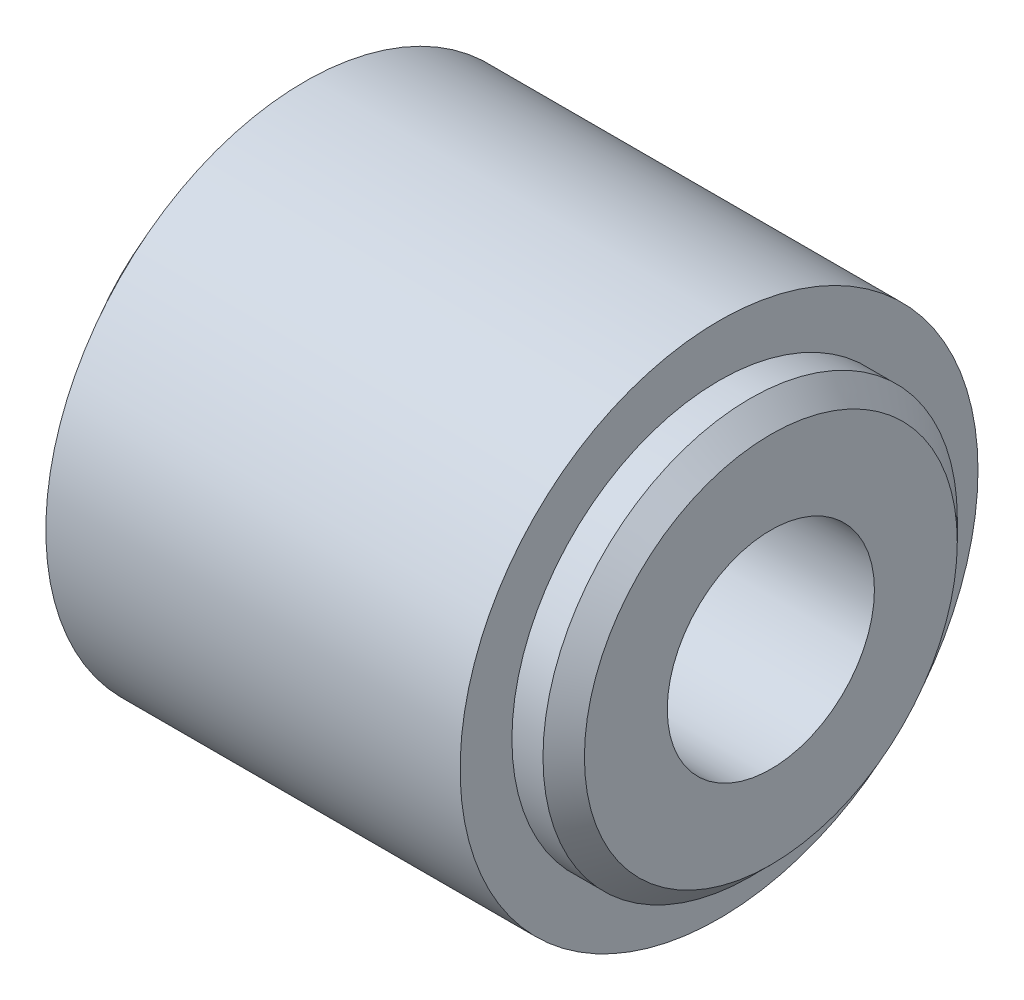
from build123d import *

# Parameters (mm, degrees)
SKETCH_1_R      = 10
SKETCH_1_R_2    = 5
EXTRUDE_1_DEPTH = 12.5
SKETCH_2_R      = 12.5
SKETCH_2_R_2    = 10
EXTRUDE_2_DEPTH = 10
CHAMFER_1_SIZE  = 1


with BuildPart() as part:
    # 草图1 → 凸台-拉伸1 (new, symmetric)
    with BuildSketch(Plane(origin=(0, 0, 0), x_dir=(0, 0, -1), z_dir=(1, 0, 0))):
        Circle(SKETCH_1_R)
        Circle(SKETCH_1_R_2, mode=Mode.SUBTRACT)
    extrude(amount=EXTRUDE_1_DEPTH, both=True)

    # 草图2 → 凸台-拉伸2 (add, symmetric)
    with BuildSketch(Plane(origin=(0, 0, 0), x_dir=(0, 0, -1), z_dir=(1, 0, 0))):
        Circle(SKETCH_2_R)
        Circle(SKETCH_2_R_2, mode=Mode.SUBTRACT)
    extrude(amount=EXTRUDE_2_DEPTH, both=True)

    # 倒角1
    chamfer_1_edges = [part.edges().sort_by_distance(p)[0] for p in [
        (-12.5, 0, 10),
        (12.5, 0, 10),
    ]]
    chamfer(chamfer_1_edges, length=CHAMFER_1_SIZE)


solid = part.part
